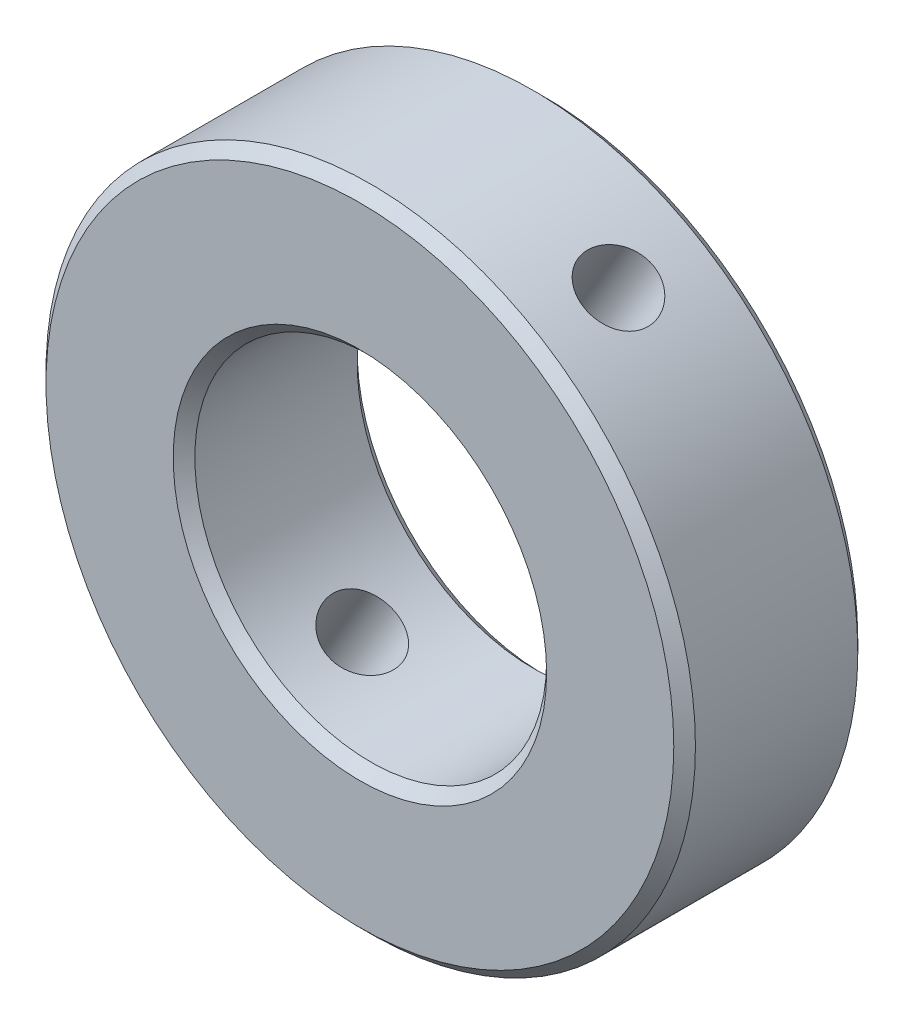
SolidWorks part; units mm, degrees
ref_plane "Front Plane" through (0, 0, 0) normal (0, 0, 1) x (1, 0, 0)
ref_plane "Top Plane" through (0, 0, 0) normal (0, 1, 0) x (1, 0, 0)
ref_plane "Right Plane" through (0, 0, 0) normal (1, 0, 0) x (0, 0, -1)
sketch "Sketch1" plane through (0, 0, 0) normal (0, 0, 1) x (1, 0, 0)
  circle A0 centre (0, 0) radius 32.5
  circle A1 centre (0, 0) radius 60
  dimension "D1" = 120
  dimension "D2" = 65
extrude "Boss-Extrude1" add sketch "Sketch1" along normal blind 34
hole_wizard "Ø13.0 (13) Diameter Hole1" positions "3DSketch1" profile "Sketch2" hole size "Ø13.0" standard "GB" end condition through all
sketch3d "3DSketch1"
  point P0 (30.8538, 51.4592, 17)
  dimension "D1" = 17
sketch "Sketch2" plane through (30.8538, 51.4592, 17) normal (0, 0, 1) x (-0.8577, 0.5142, 0)
  line L0 (0, 0) -> (0, 142.3129)
  line L1 (0, 142.3129) -> (6.5, 142.3129)
  line L2 (6.5, 142.3129) -> (6.5, 0)
  line L5 (6.5, 0) -> (0, 0)
  line L11 (0, -6.35) -> (0, 107.95) construction
  dimension "通孔孔直径" = 13
  dimension "通孔孔深度" = 142.3129
chamfer "Chamfer1" distance 2 angle 45 4 edges at (60, 0, 0) (60, 0, 34) (32.5, 0, 0) (32.5, 0, 34)
